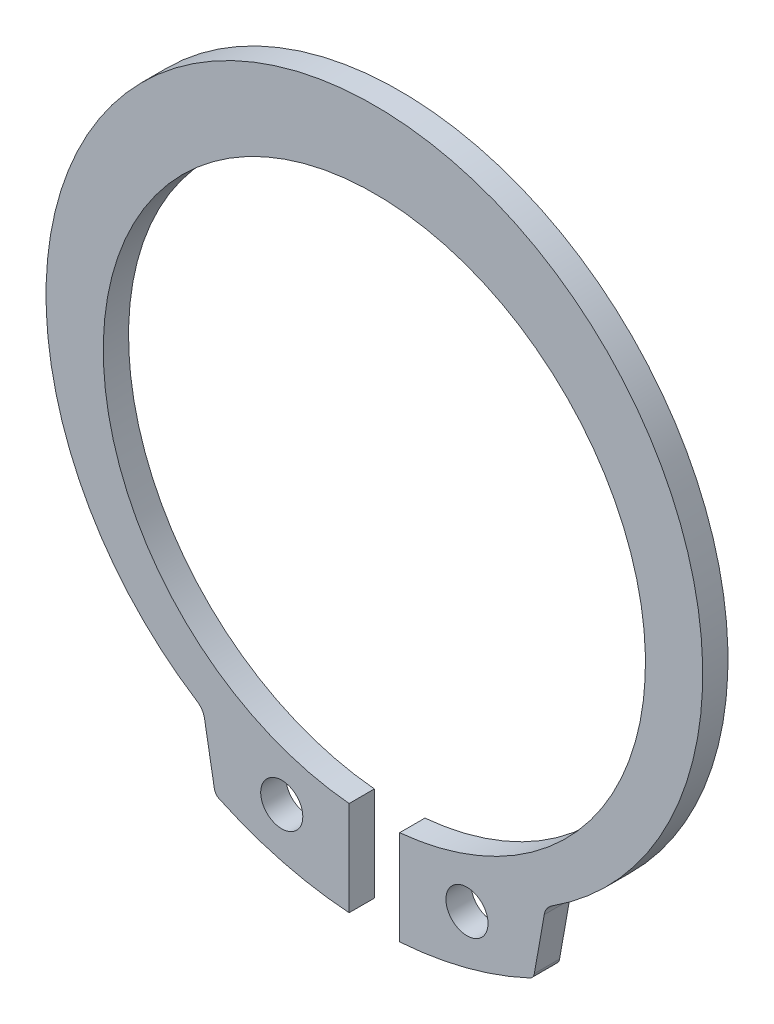
from build123d import *

# Parameters (mm, degrees)
BASE_EXTRUDE_DEPTH      = 0.75
BASE_EXTRUDE_DEPTH_BACK = 0.75
SKETCH1_R               = 1.25


with BuildPart() as part:
    # Sketch1 → Base-Extrude (new, two sides: drawn at the far end of the back side and taken through both)
    with BuildSketch(Plane.XY.offset(-BASE_EXTRUDE_DEPTH_BACK)):
        with BuildLine():
            Line((-1.5, -17.159971928), (-1.5, -22.778094604))
            ThreePointArc((-1.5, -22.778094604), (-5.452894614, -22.133712537), (-9.220039428, -20.773850767))
            ThreePointArc((-9.220039428, -20.773850767), (-9.404653614, -20.625111252), (-9.5, -20.408051566))
            Line((-9.5, -20.408051566), (-10.086937259, -17.079364962))
            ThreePointArc((-10.086937259, -17.079364962), (-10.239358111, -16.698818185), (-10.531659889, -16.411402743))
            ThreePointArc((-10.531659889, -16.411402743), (0, 19.5), (10.531659889, -16.411402743))
            ThreePointArc((10.531659889, -16.411402743), (10.239358111, -16.698818185), (10.086937259, -17.079364962))
            Line((10.086937259, -17.079364962), (9.5, -20.408051566))
            ThreePointArc((9.5, -20.408051566), (9.404653614, -20.625111252), (9.220039428, -20.773850767))
            ThreePointArc((9.220039428, -20.773850767), (5.452894614, -22.133712537), (1.5, -22.778094604))
            Line((1.5, -22.778094604), (1.5, -17.159971928))
            ThreePointArc((1.5, -17.159971928), (0, 14.97), (-1.5, -17.159971928))
        make_face()
        with Locations((-5.5, -19.212035284)):
            Circle(SKETCH1_R, mode=Mode.SUBTRACT)
        with Locations(Location((5.5, -19.212035284, 0), (0, 0, 180))):
            Circle(SKETCH1_R, mode=Mode.SUBTRACT)
    extrude(amount=BASE_EXTRUDE_DEPTH + BASE_EXTRUDE_DEPTH_BACK)


solid = part.part
